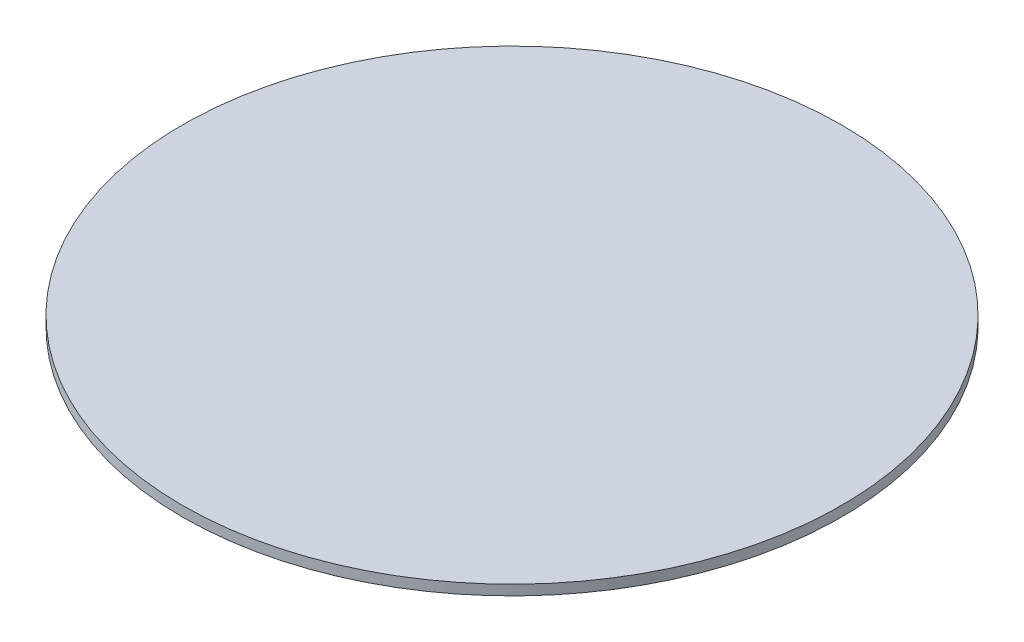
from build123d import *

# Parameters (mm, degrees)
SKETCH1_R           = 32.5
BOSS_EXTRUDE1_DEPTH = 1


with BuildPart() as part:
    # Sketch1 → Boss-Extrude1 (new body)
    with BuildSketch(Plane(origin=(0, 0, 0), x_dir=(1, 0, 0), z_dir=(0, 1, 0))):
        with Locations(Location((0, 0, 0), (0, 0, 270))):
            Circle(SKETCH1_R)
    extrude(amount=BOSS_EXTRUDE1_DEPTH)


solid = part.part
